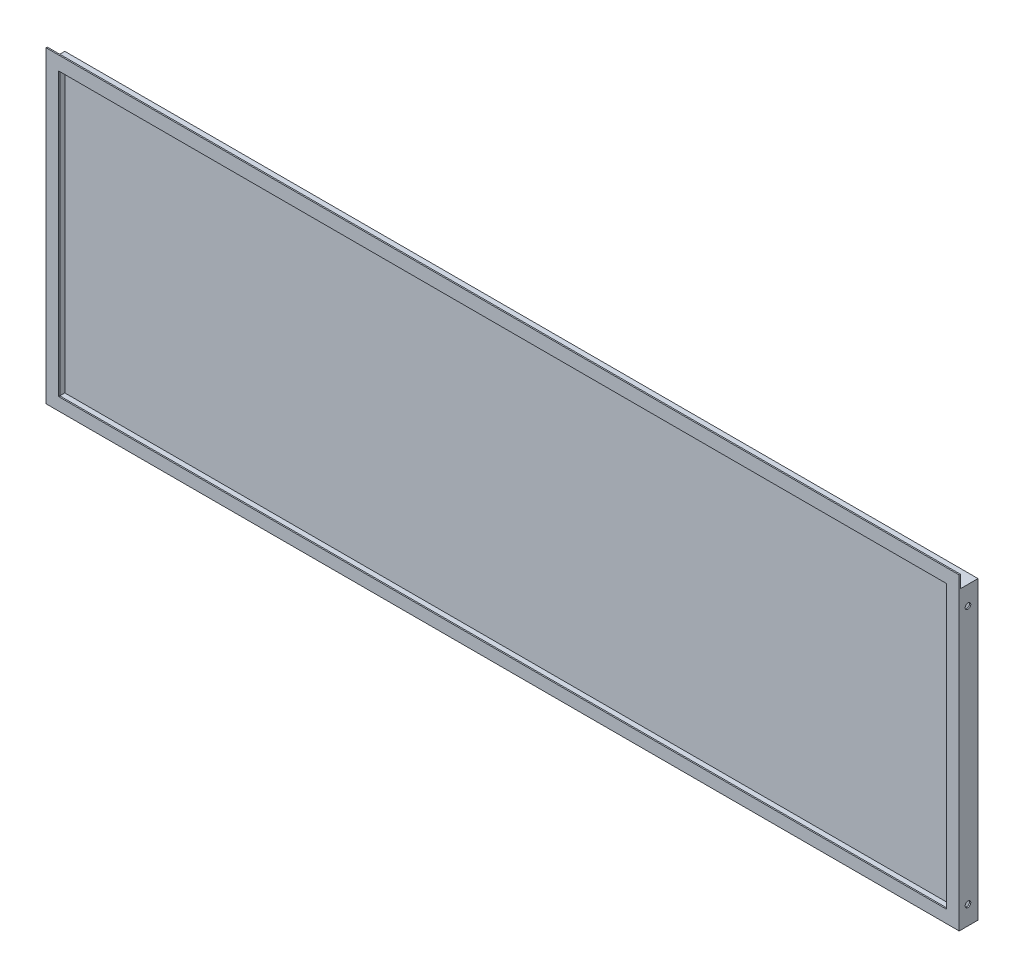
SolidWorks part; units mm, degrees
ref_plane "前视基准面" through (0, 0, 0) normal (0, 0, 1) x (1, 0, 0)
ref_plane "上视基准面" through (0, 0, 0) normal (0, 1, 0) x (1, 0, 0)
ref_plane "右视基准面" through (0, 0, 0) normal (1, 0, 0) x (0, 0, -1)
sketch "草图1" plane through (0, 0, 0) normal (0, 0, 1) x (1, 0, 0)
  line L1 (0, 0) -> (1457, 0)
  line L2 (0, 0) -> (0, 472)
  line L3 (0, 472) -> (1457, 472)
  line L4 (1457, 0) -> (1457, 472)
  dimension "D1" = 472
  dimension "D2" = 1457
extrude "凸台-拉伸1" add sketch "草图1" along normal blind 30
shell "抽壳1" thickness 2
sketch "草图2" plane through (0, 0, 30) normal (0, 0, 1) x (1, 0, 0)
  line L0 (1455, 470) -> (2, 470) construction
  line L1 (0, 492) -> (1457, 492)
  line L2 (0, 492) -> (0, 0)
  line L3 (0, 0) -> (1457, 0)
  line L4 (1457, 492) -> (1457, 0)
  line L5 (0, 472) -> (0, 0) construction
  line L6 (1457, 472) -> (0, 472) construction
  line L7 (1455, 470) -> (2, 470) construction
  line L8 (20, 20) -> (1437, 20)
  line L9 (20, 20) -> (20, 470)
  line L10 (20, 470) -> (1437, 470)
  line L11 (1437, 20) -> (1437, 470)
  dimension "D1" = 20
  dimension "D2" = 20
  dimension "D3" = 20
  dimension "D4" = 20
extrude "凸台-拉伸2" add sketch "草图2" against normal blind 2
sketch "草图3" plane through (2, 0, 0) normal (1, 0, 0) x (0, 0, -1)
  line L0 (-16, 493.0591) -> (-16, -33.6571) construction
  line L4 (-30, 0) -> (-30, 492) construction
  line L5 (-30, 0) -> (0, 0) construction
  line L6 (-28, 472) -> (0, 472) construction
  circle A0 centre (-16, 442) radius 4.5
  circle A1 centre (-16, 30) radius 4.5
  dimension "D2" = 9
  dimension "D3" = 9
  dimension "D4" = 30
  dimension "D5" = 30
  dimension "D1" = 14
extrude "切除-拉伸1" cut sketch "草图3" against normal blind 10 and the other way blind 1501
sketch "草图6" plane through (0, 2, 0) normal (0, 1, 0) x (1, 0, 0)
  line L0 (-41.0114, -16) -> (1543.1613, -16) construction
  line L1 (0, -30) -> (1457, -30) construction
  line L2 (0, -30) -> (0, 0) construction
  line L3 (1457, -28) -> (1457, 0) construction
  circle A0 centre (30, -16) radius 4.5
  circle A1 centre (450, -16) radius 4.5
  circle A2 centre (1427, -16) radius 4.5
  circle A3 centre (968.5, -16) radius 4.5
  circle A4 centre (510, -16) radius 4.5
  circle A5 centre (78, -16) radius 4.5
  circle A6 centre (178, -16) radius 4.5
  dimension "D2" = 9
  dimension "D3" = 30
  dimension "D4" = 9
  dimension "D5" = 450
  dimension "D6" = 9
  dimension "D7" = 30
  dimension "D8" = 9
  dimension "D9" = 9
  dimension "D10" = 60
  dimension "D11" = 458.5
  dimension "D12" = 9
  dimension "D13" = 9
  dimension "D14" = 100
  dimension "D15" = 78
  dimension "D1" = 14
extrude "切除-拉伸2" cut sketch "草图6" against normal blind 10
